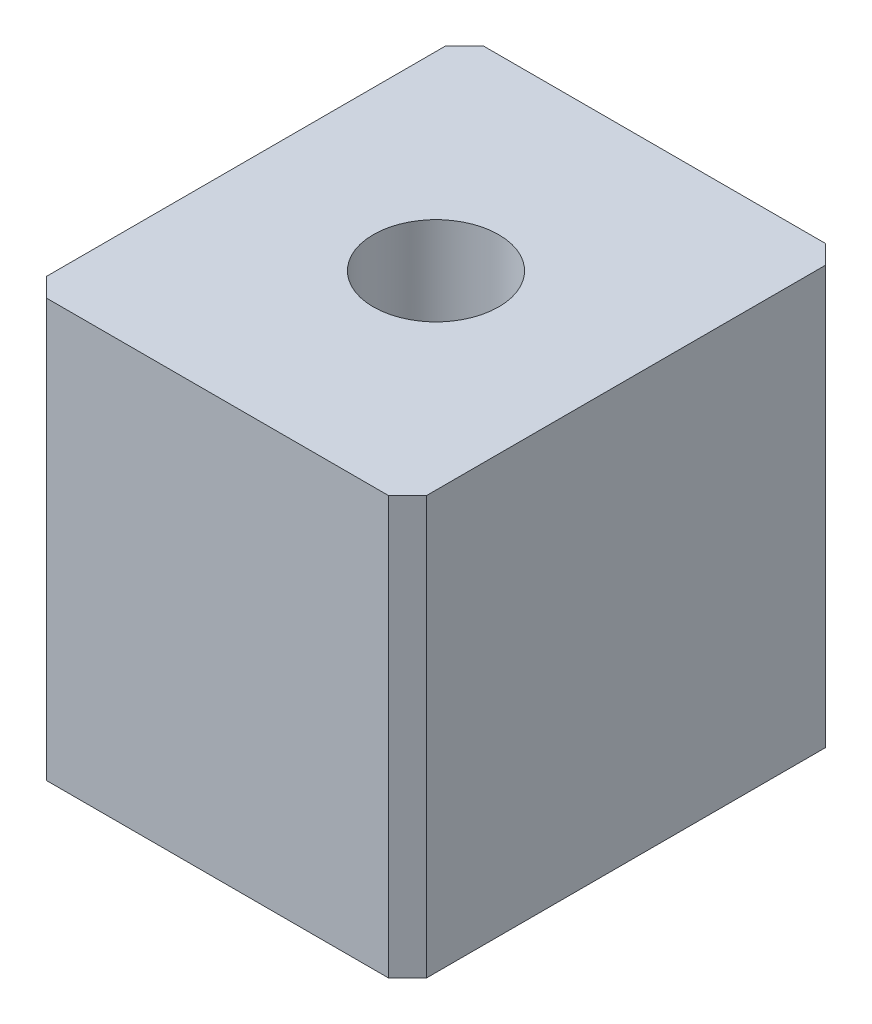
from build123d import *

# Parameters (mm, degrees)
SKETCH_1_W                   = 20
SKETCH_1_H                   = 23
EXTRUDE_1_DEPTH              = 22
HOLE_WIZARD_M6_1_D           = 6.6
HOLE_WIZARD_M6_1_DEPTH       = 22.25
HOLE_WIZARD_M6_1_CBORE_D     = 11
HOLE_WIZARD_M6_1_CBORE_DEPTH = 15
HOLE_WIZARD_M6_1_TIP         = 1.982840043
CHAMFER_1_SIZE               = 1


with BuildPart() as part:
    # 草图1 → 凸台-拉伸1 (new body)
    with BuildSketch(Plane(origin=(0, 0, 0), x_dir=(1, 0, 0), z_dir=(0, 1, 0))):
        Rectangle(SKETCH_1_W, SKETCH_1_H)
    extrude(amount=EXTRUDE_1_DEPTH)

    # M6 六角凹头螺钉的柱形沉头孔1
    with Locations(Plane(origin=(0, 0, 0), x_dir=(-1, 0, 0), z_dir=(0, -1, 0))):
        with Locations((0, 0)):
            CounterBoreHole(HOLE_WIZARD_M6_1_D / 2, HOLE_WIZARD_M6_1_CBORE_D / 2, HOLE_WIZARD_M6_1_CBORE_DEPTH, depth=HOLE_WIZARD_M6_1_DEPTH)
            with Locations((0, 0, -(HOLE_WIZARD_M6_1_DEPTH + HOLE_WIZARD_M6_1_TIP / 2))):  # 118° drill point
                Cone(0, HOLE_WIZARD_M6_1_D / 2, HOLE_WIZARD_M6_1_TIP, mode=Mode.SUBTRACT)

    # 倒角1
    chamfer_1_edges = [part.edges().sort_by_distance(p)[0] for p in [
        (10, 11, 11.5),
        (-10, 11, 11.5),
        (-10, 11, -11.5),
        (10, 11, -11.5),
    ]]
    chamfer(chamfer_1_edges, length=CHAMFER_1_SIZE)


solid = part.part
